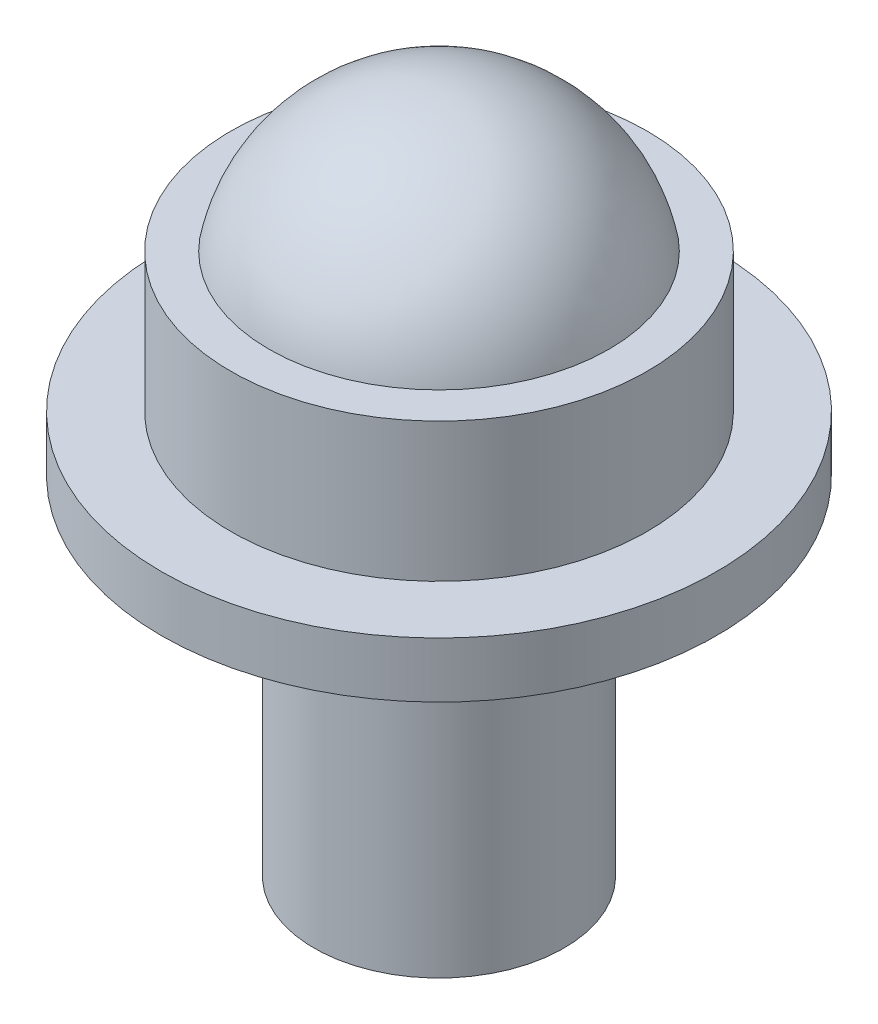
SolidWorks part; units mm, degrees
material "AISI 1015 钢，冷拔 (SS)"
ref_plane "Front Plane" through (0, 0, 0) normal (0, 0, 1) x (1, 0, 0)
ref_plane "Top Plane" through (0, 0, 0) normal (0, 1, 0) x (1, 0, 0)
ref_plane "Right Plane" through (0, 0, 0) normal (1, 0, 0) x (0, 0, -1)
other "Configuration Table"
sketch "Sketch1" plane through (0, 0, 0) normal (0, 0, 1) x (1, 0, 0)
  line L0 (0, 0) -> (0, 59.0607) construction
  line L1 (-24.4949, 28) -> (-30, 28)
  line L2 (-30, 28) -> (-30, 8)
  line L3 (-30, 8) -> (-40, 8)
  line L4 (-40, 8) -> (-40, 0)
  line L5 (-40, 0) -> (0, 0)
  line L6 (0, 0) -> (0, 48)
  arc A0 (0, 48) -> (-24.4949, 28) centre (0, 23) ccw
  dimension "D6" = 25
  dimension "D1" = 20
  dimension "D2" = 8
  dimension "D3" = 40
  dimension "D4" = 30
  dimension "D5" = 20
revolve "Revolve1" add sketch "Sketch1" angle 360 about L0
sketch "Sketch2" plane through (0, 0, 0) normal (0, -1, 0) x (-1, 0, 0)
  circle A0 centre (0, 0) radius 18
  dimension "D1" = 36
extrude "Boss-Extrude1" add sketch "Sketch2" along normal blind 50
